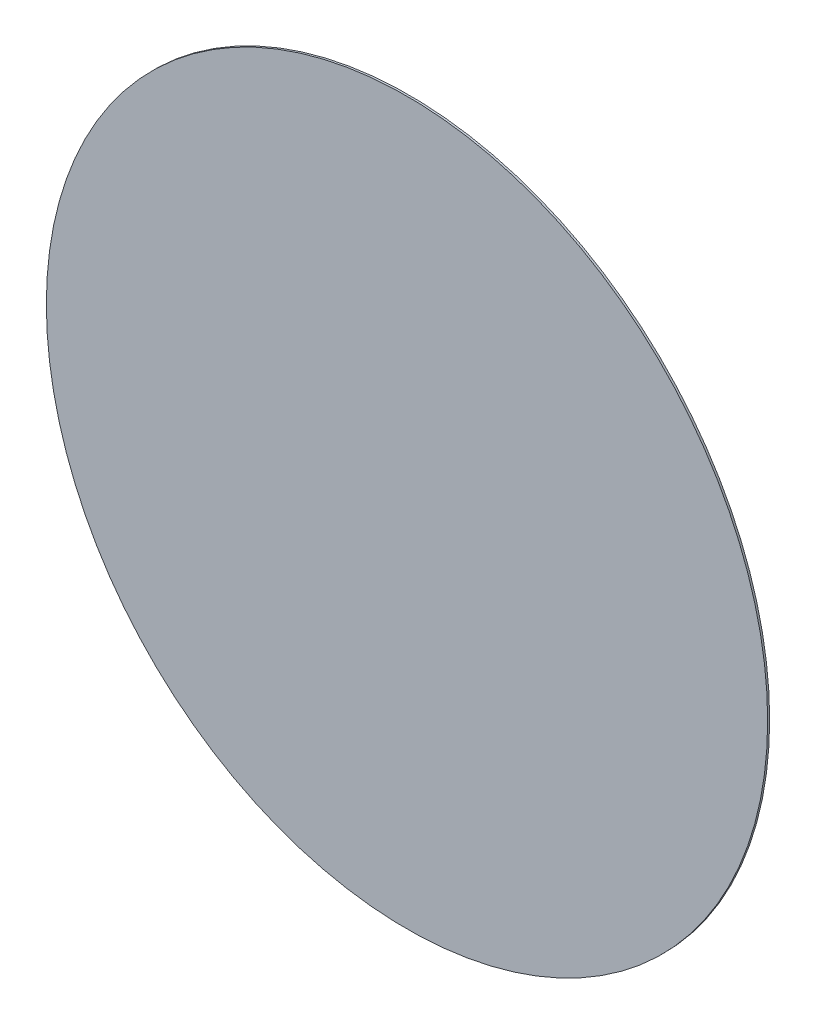
from build123d import *

# Parameters (mm, degrees)
SKETCH_1_R      = 54
EXTRUDE_1_DEPTH = 0.3


with BuildPart() as part:
    # 草图1 → 凸台-拉伸1 (new body)
    with BuildSketch(Plane.XY):
        Circle(SKETCH_1_R)
    extrude(amount=EXTRUDE_1_DEPTH)


solid = part.part
